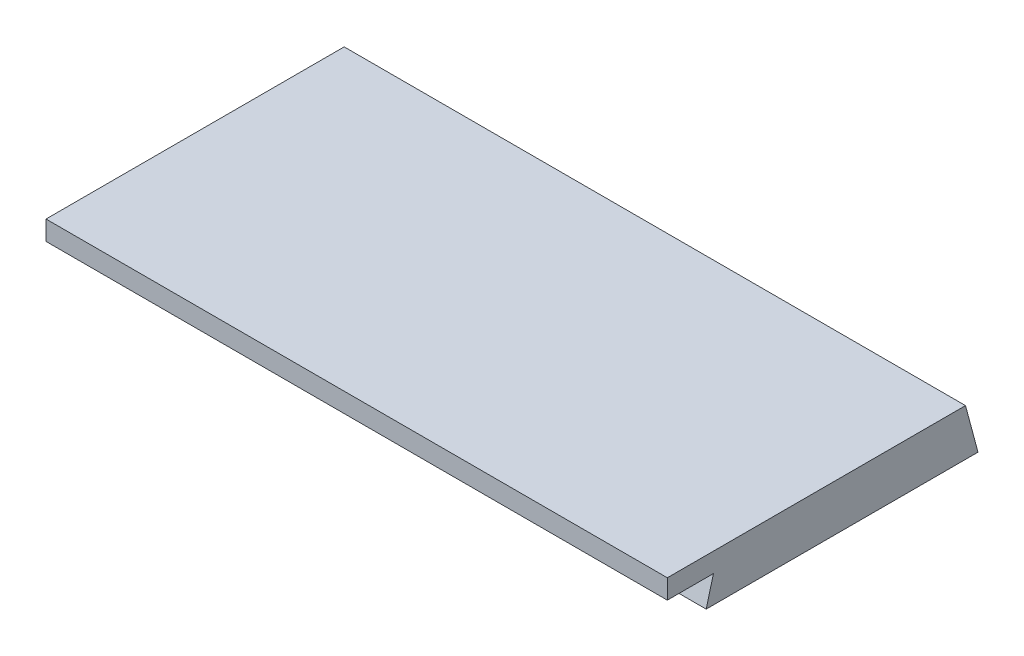
from build123d import *

# Parameters (mm, degrees)
BOSS_EXTRUDE1_DEPTH = 400


with BuildPart() as part:
    # Sketch1 → Boss-Extrude1 (new, symmetric)
    with BuildSketch(Plane(origin=(0, 0, 0), x_dir=(0, 0, -1), z_dir=(1, 0, 0))):
        Polygon((350, 0), (333.923048454, 60), (-50, 60), (-50, 35), (9.378221735, 35), (0, 0), align=None)
    extrude(amount=BOSS_EXTRUDE1_DEPTH, both=True)


solid = part.part
